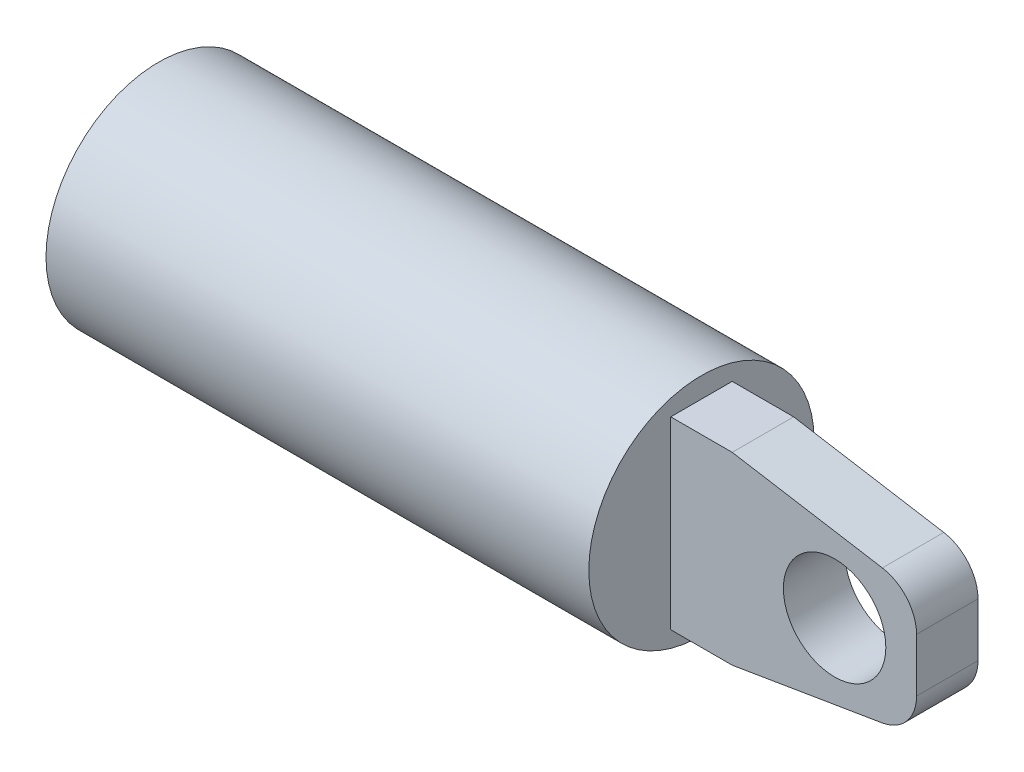
SolidWorks part; units mm, degrees
ref_plane "Front Plane" through (0, 0, 0) normal (0, 0, 1) x (1, 0, 0)
ref_plane "Top Plane" through (0, 0, 0) normal (0, 1, 0) x (1, 0, 0)
ref_plane "Right Plane" through (0, 0, 0) normal (1, 0, 0) x (0, 0, -1)
sketch "Sketch1" plane through (0, 0, 0) normal (0, 0, 1) x (1, 0, 0)
  line L0 (0, 11) -> (0, 0)
  line L1 (0, 0) -> (53, 0)
  line L2 (53, 0) -> (53, 11)
  line L3 (53, 11) -> (0, 11)
  line L4 (0, 0) -> (53, 0) construction
revolve "Revolve1" add sketch "Sketch1" angle 360 about L4
ref_plane "Plane1" through (0, 0, 3) normal (0, 0, 1) x (1, 0, 0)
sketch "Sketch2" plane through (0, 0, 3) normal (0, 0, 1) x (1, 0, 0)
  line L0 (77, -6) -> (77, 6)
  line L1 (77, 6) -> (59, 9)
  line L2 (59, 9) -> (53, 9)
  line L3 (53, 9) -> (53, -9)
  line L4 (53, -9) -> (59, -9)
  line L5 (59, -9) -> (77, -6)
extrude "Boss-Extrude1" add sketch "Sketch2" against normal blind 6
hole_wizard "Ø10.0 (10) Diameter Hole1" positions "Sketch4" profile "Sketch3" hole size "Ø10.0" standard "ANSI Metric"
sketch "Sketch4" plane through (0, 0, -3) normal (0, 0, -1) x (-1, 0, 0)
  point P0 (-69, 0)
sketch "Sketch3" plane through (69, 0, -3) normal (1, 0, 0) x (0, 1, 0)
  line L0 (0, 0) -> (0, 14)
  line L1 (0, 14) -> (5, 14)
  line L2 (5, 14) -> (5, 0)
  line L5 (5, 0) -> (0, 0)
  line L11 (0, -6.35) -> (0, 107.95) construction
  dimension "通孔孔直径" = 10
  dimension "通孔孔深度" = 14
hole_wizard "CBORE for M13 SHSS1" positions "Sketch6" profile "Sketch5" counterbore size "M13" standard "ANSI Metric"
sketch "Sketch6" plane through (0, 0, 0) normal (-1, 0, 0) x (0, 0, 1)
  point P0 (0, 0)
sketch "Sketch5" plane through (0, 0, 0) normal (0, 1, 0) x (0, 0, 1)
  line L0 (0, 0) -> (0, 50)
  line L1 (0, 50) -> (8, 50)
  line L2 (8, 50) -> (8, 5)
  line L3 (8, 5) -> (4, 5)
  line L4 (4, 5) -> (4, 0)
  line L5 (4, 0) -> (0, 0)
  line L10 (0, 50) -> (-8, 50) construction
  line L11 (0, -6.35) -> (0, 107.95) construction
  dimension "孔直径" = 16
  dimension "孔深度" = 50
  dimension "柱形沉头孔直径" = 8
  dimension "柱形沉头孔深度" = 5
  dimension "导头角度" = 180
fillet "Fillet1" radius 4 2 edges at (77, 6, 0) (77, -6, 0)
